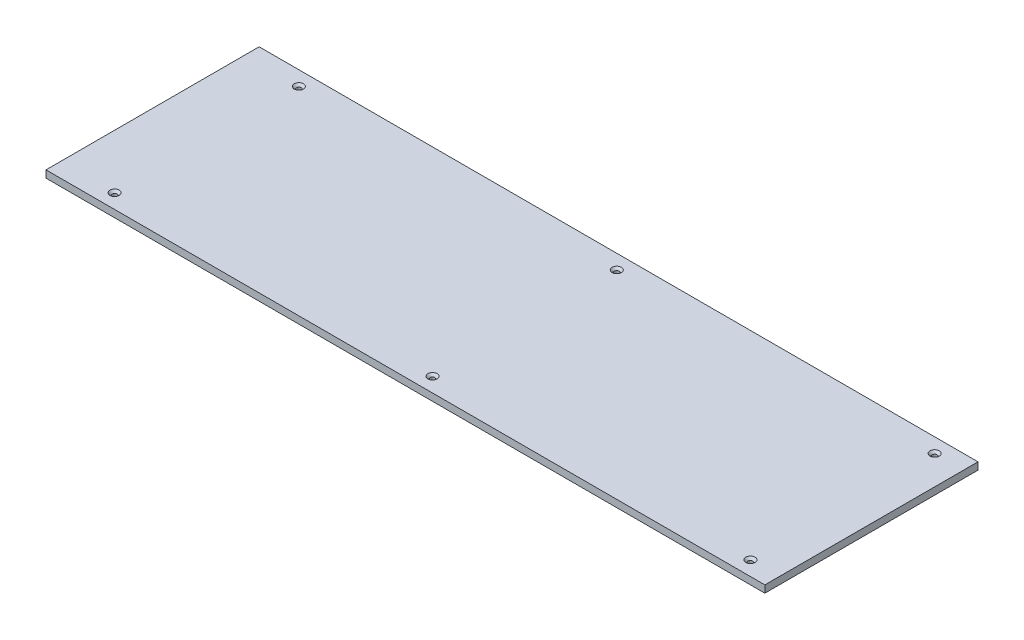
from build123d import *

# Parameters (mm, degrees)
SKETCH1_W                                         = 995
SKETCH1_H                                         = 295
BOSS_EXTRUDE1_DEPTH                               = 10
HOLE_SIZE_BASED_HEXALOBULAR_SOCKET_SE_D           = 6.6
HOLE_SIZE_BASED_HEXALOBULAR_SOCKET_SE_DEPTH       = 19.75
HOLE_SIZE_BASED_HEXALOBULAR_SOCKET_SE_CSINK_D     = 12.8
HOLE_SIZE_BASED_HEXALOBULAR_SOCKET_SE_CSINK_ANGLE = 90
HOLE_SIZE_BASED_HEXALOBULAR_SOCKET_SE_TIP         = 1.982840043


with BuildPart() as part:
    # Sketch1 → Boss-Extrude1 (new body)
    with BuildSketch(Plane(origin=(0, 0, 0), x_dir=(1, 0, 0), z_dir=(0, 1, 0))):
        with Locations((497.5, -147.5)):
            Rectangle(SKETCH1_W, SKETCH1_H)
    extrude(amount=BOSS_EXTRUDE1_DEPTH)

    # Hole Size (% based) Hexalobular Socket Semi-Countersunk Screw Type1
    with Locations(Plane(origin=(0, 10, 0), x_dir=(1, 0, 0), z_dir=(0, 1, 0))):
        with Locations((75, -20), (75, -275), (515, -20), (515, -275), (955, -275), (955, -20)):
            CounterSinkHole(HOLE_SIZE_BASED_HEXALOBULAR_SOCKET_SE_D / 2, HOLE_SIZE_BASED_HEXALOBULAR_SOCKET_SE_CSINK_D / 2, depth=HOLE_SIZE_BASED_HEXALOBULAR_SOCKET_SE_DEPTH, counter_sink_angle=HOLE_SIZE_BASED_HEXALOBULAR_SOCKET_SE_CSINK_ANGLE)
            with Locations((0, 0, -(HOLE_SIZE_BASED_HEXALOBULAR_SOCKET_SE_DEPTH + HOLE_SIZE_BASED_HEXALOBULAR_SOCKET_SE_TIP / 2))):  # 118° drill point
                Cone(0, HOLE_SIZE_BASED_HEXALOBULAR_SOCKET_SE_D / 2, HOLE_SIZE_BASED_HEXALOBULAR_SOCKET_SE_TIP, mode=Mode.SUBTRACT)


solid = part.part
